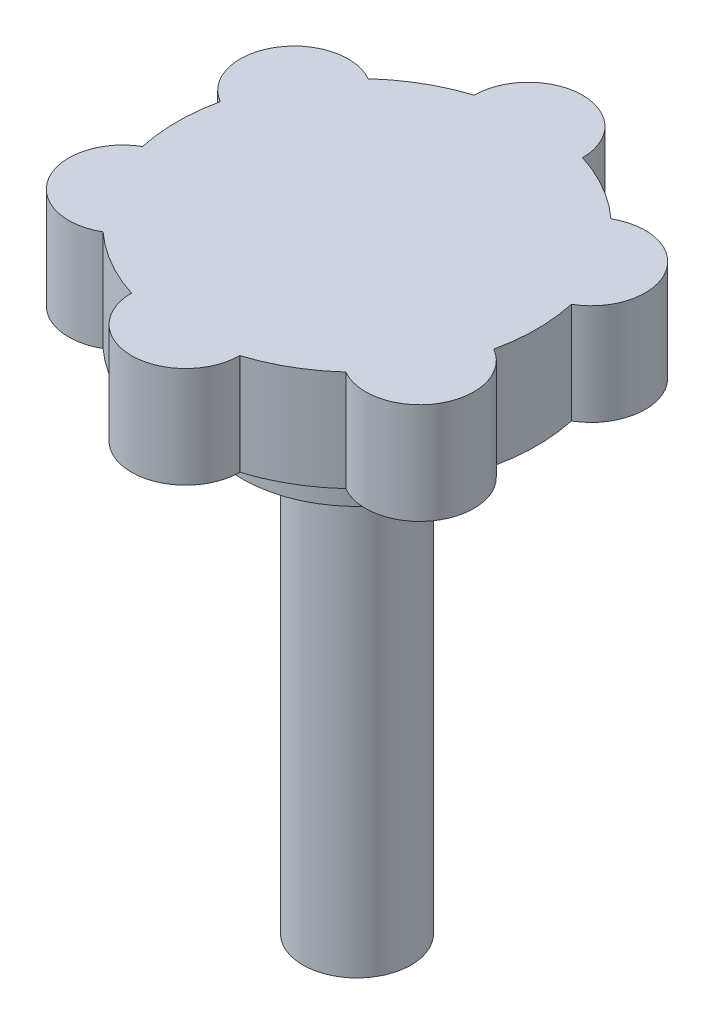
from build123d import *

# Parameters (mm, degrees)
BOSS_EXTRUDE1_DEPTH = 5.6
SKETCH2_R           = 6.35
BOSS_EXTRUDE2_DEPTH = 3.4
SKETCH3_R           = 3
BOSS_EXTRUDE3_DEPTH = 25


with BuildPart() as part:
    # Sketch1 → Boss-Extrude1 (new body)
    with BuildSketch(Plane(origin=(0, 0, 0), x_dir=(1, 0, 0), z_dir=(0, 1, 0))):
        with BuildLine():
            Line((-9.72424134, -2.15192377), (-9.725740285, -2.152789186))
            ThreePointArc((-9.725740285, -2.152789186), (-10.823817926, -6.250865027), (-6.725742085, -7.348942669))
            Line((-6.725742085, -7.348942669), (-6.723420775, -7.34760246))
            ThreePointArc((-6.723420775, -7.34760246), (-4.978167749, -8.626268935), (-2.998, -9.497952231))
            Line((-2.998, -9.497952231), (-2.998, -9.5))
            ThreePointArc((-2.998, -9.5), (0.002000003, -12.499999996), (3.002, -9.499999993))
            Line((3.002, -9.499999993), (3.002, -9.497636397))
            ThreePointArc((3.002, -9.497636397), (4.982303032, -8.625613539), (6.727581168, -7.346540363))
            Line((6.727581168, -7.346540363), (6.728741336, -7.347210186))
            ThreePointArc((6.728741336, -7.347210186), (10.826817547, -6.249133975), (9.728741336, -2.151057763))
            Line((9.728741336, -2.151057763), (9.727581168, -2.15038794))
            ThreePointArc((9.727581168, -2.15038794), (9.962651964, 0.001128196), (9.727467916, 2.152631955))
            ThreePointArc((9.727467916, 2.152631955), (10.825817547, 6.250866025), (6.727194396, 7.348626461))
            ThreePointArc((6.727194396, 7.348626461), (4.981167779, 8.628000969), (3, 9.5))
            ThreePointArc((3, 9.5), (2e-09, 12.5), (-3, 9.499052498))
            ThreePointArc((-3, 9.499052498), (-4.980665222, 8.626558938), (-6.726128008, 7.346856081))
            ThreePointArc((-6.726128008, 7.346856081), (-10.824817547, 6.249133975), (-9.726741336, 2.151057764))
            Line((-9.726741336, 2.151057764), (-9.725033927, 2.150071991))
            ThreePointArc((-9.725033927, 2.150071991), (-9.959651798, -0.000969188), (-9.72424134, -2.15192377))
        make_face()
    extrude(amount=BOSS_EXTRUDE1_DEPTH)

    # Sketch2 → Boss-Extrude2 (add)
    with BuildSketch(Plane.XZ):
        with Locations(Location((0, 0, 0), (0, 0, 90))):
            Circle(SKETCH2_R)
    extrude(amount=BOSS_EXTRUDE2_DEPTH)

    # Sketch3 → Boss-Extrude3 (add)
    with BuildSketch(Plane.XZ.offset(3.4)):
        with Locations(Location((0, 0, 0), (0, 0, 270))):
            Circle(SKETCH3_R)
    extrude(amount=BOSS_EXTRUDE3_DEPTH)


solid = part.part
